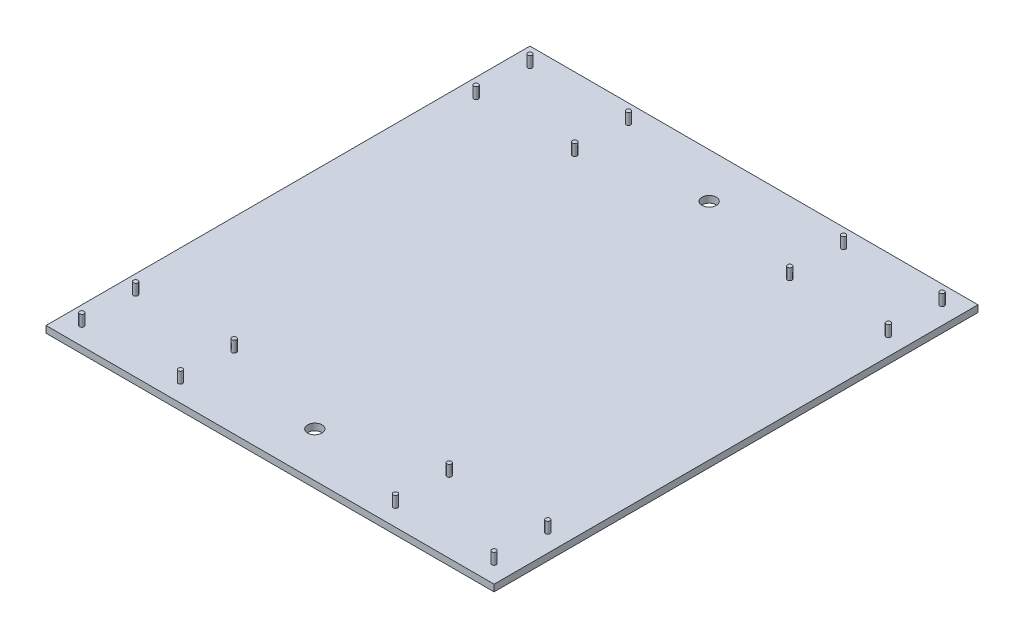
SolidWorks part; units mm, degrees
ref_plane "Front Plane" through (0, 0, 0) normal (0, 0, 1) x (1, 0, 0)
ref_plane "Top Plane" through (0, 0, 0) normal (0, 1, 0) x (1, 0, 0)
ref_plane "Right Plane" through (0, 0, 0) normal (1, 0, 0) x (0, 0, -1)
other "Configuration Table"
sketch "Sketch1" plane through (0, 0, 0) normal (0, 1, 0) x (1, 0, 0)
  line L1 (-1000, -1080) -> (1000, -1080)
  line L2 (-1000, -1080) -> (-1000, 1080)
  line L3 (-1000, 1080) -> (1000, 1080)
  line L4 (1000, -1080) -> (1000, 1080)
  line L5 (-1000, -1080) -> (1000, 1080) construction
  line L6 (-1000, 1080) -> (1000, -1080) construction
  point P0 (0, 0)
  dimension "D1" = 2000
  dimension "D2" = 2160
extrude "Boss-Extrude1" add sketch "Sketch1" along normal blind 30
ref_plane "Plane2" through (0, 0, 0) normal (1, 0, 0) x (0, 0, -1)
sketch "Sketch2" plane through (0, 30, 0) normal (0, 1, 0) x (1, 0, 0)
  line L0 (1000, 1080) -> (-1000, 1080) construction
  line L1 (-1000, 1080) -> (-1000, -1080) construction
  line L2 (0, 1080) -> (0, -1092.2464) construction
  line L3 (0, -16.5) -> (0, 16.5) construction
  line L4 (-1000, 0) -> (1000, 0) construction
  line L5 (1000, -1080) -> (1000, 1080) construction
  circle A0 centre (-920, 1000) radius 10
  circle A1 centre (-920, 760) radius 10
  circle A2 centre (-480, 1000) radius 10
  circle A3 centre (-480, 760) radius 10
  circle A4 centre (480, 760) radius 10
  circle A5 centre (480, 1000) radius 10
  circle A6 centre (920, 760) radius 10
  circle A7 centre (920, 1000) radius 10
  circle A8 centre (920, -1000) radius 10
  circle A9 centre (920, -760) radius 10
  circle A10 centre (480, -1000) radius 10
  circle A11 centre (480, -760) radius 10
  circle A12 centre (-480, -760) radius 10
  circle A13 centre (-480, -1000) radius 10
  circle A14 centre (-920, -760) radius 10
  circle A15 centre (-920, -1000) radius 10
  dimension "D1" = 20
  dimension "D3" = 80
  dimension "D4" = 20
  dimension "D6" = 80
  dimension "D7" = 20
  dimension "D9" = 80
  dimension "D10" = 20
  dimension "D11" = 240
  dimension "D12" = 440
  dimension "D2" = 80
  dimension "D5" = 240
  dimension "D8" = 440
extrude "Boss-Extrude2" add sketch "Sketch2" along normal blind 50
cosmetic thread "Cosmetic Thread1" parameters "D2"=19
cosmetic thread "Cosmetic Thread2" parameters "D2"=19
cosmetic thread "Cosmetic Thread3" parameters "D2"=19
cosmetic thread "Cosmetic Thread4" parameters "D2"=19
cosmetic thread "Cosmetic Thread5" parameters "D2"=19
cosmetic thread "Cosmetic Thread6" parameters "D2"=19
cosmetic thread "Cosmetic Thread7" parameters "D2"=19
cosmetic thread "Cosmetic Thread8" parameters "D2"=19
cosmetic thread "Cosmetic Thread9" parameters "D2"=19
cosmetic thread "Cosmetic Thread10" parameters "D2"=19
cosmetic thread "Cosmetic Thread11" parameters "D2"=19
cosmetic thread "Cosmetic Thread12" parameters "D2"=19
cosmetic thread "Cosmetic Thread13" parameters "D2"=19
cosmetic thread "Cosmetic Thread14" parameters "D2"=19
cosmetic thread "Cosmetic Thread15" parameters "D2"=19
cosmetic thread "Cosmetic Thread16" parameters "D2"=19
sketch "Sketch3" plane through (0, 30, 0) normal (0, 1, 0) x (1, 0, 0)
  line L0 (0, 1080) -> (0, -1080) construction
  line L1 (1000, 1080) -> (-1000, 1080) construction
  line L2 (-1000, -1080) -> (1000, -1080) construction
  circle A0 centre (0, 880) radius 32
  circle A1 centre (0, -880) radius 32
  dimension "D2" = 64
  dimension "D3" = 64
  dimension "D1" = 200
  dimension "D4" = 200
extrude "Cut-Extrude1" cut sketch "Sketch3" against normal blind 40
